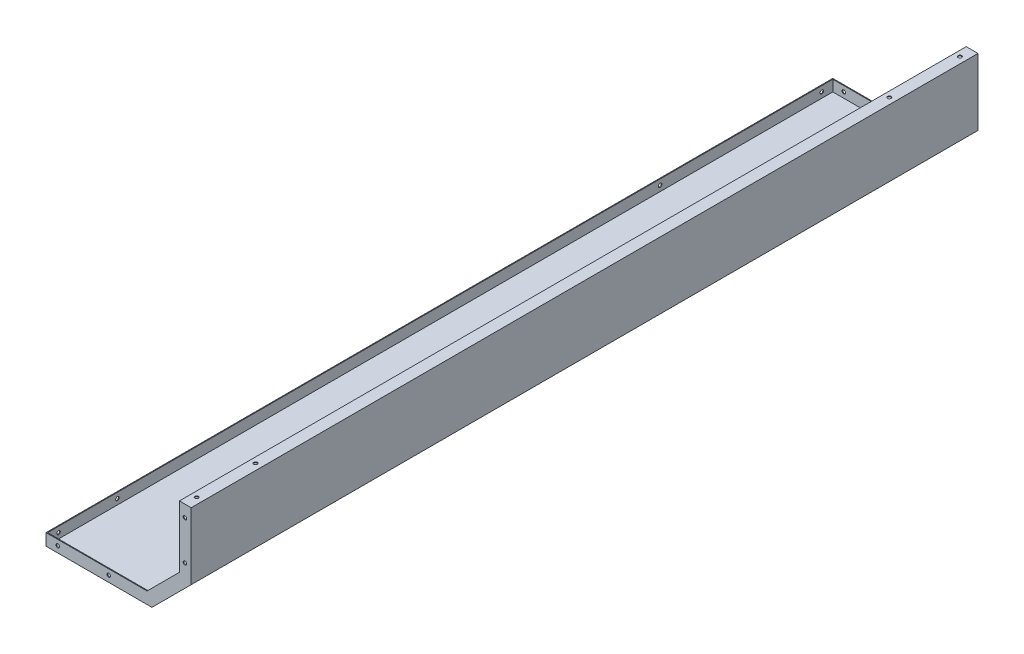
from build123d import *

# Parameters (mm, degrees)
EXTRUDE_1_DEPTH          = 2005
EXTRUDE_1_2_DEPTH        = 28
SKETCH_5_W               = 2
SKETCH_5_H               = 139.764501988
EXTRUDE_2_DEPTH          = 28
SKETCH_6_W               = 269.171572875
SKETCH_6_H               = 2
EXTRUDE_3_DEPTH          = 28
SKETCH_7_W               = 2
SKETCH_7_H               = 2005
EXTRUDE_4_DEPTH          = 28
CUT_EXTRUDE_1_DEPTH      = 10
CUT_EXTRUDE_1_DEPTH_BACK = 10
SKETCH_8_R               = 4.5
SKETCH_9_R               = 4.5
CUT_EXTRUDE_2_DEPTH      = 10
SKETCH_10_R              = 4.5
CUT_EXTRUDE_3_DEPTH      = 76
SKETCH_11_R              = 4.5
CUT_EXTRUDE_4_DEPTH      = 63
SKETCH_12_R              = 4.5
CUT_EXTRUDE_5_DEPTH      = 10
SKETCH_13_R              = 4.5
CUT_EXTRUDE_6_DEPTH      = 10


with BuildPart() as part:
    # 草图1 → Extrude 1 (new body)
    with BuildSketch(Plane.XY):
        Polygon((0, 0), (270, 0), (370, 100), (370, 270), (368, 270), (368, 100.828427125), (269.171572875, 2), (0, 2), align=None)
    extrude(amount=EXTRUDE_1_DEPTH)

    # 草图4 → Extrude 1 2 (add)
    with BuildSketch(Plane.ZY.offset(-368)):
        Polygon((0, 100.828427125), (0, 270), (2005, 270), (2005, 100.828427125), (2003, 100.828427125), (2003, 268), (2, 268), (2, 100.828427125), align=None)
    extrude(amount=EXTRUDE_1_2_DEPTH)

    # 草图5 → 凸台-拉伸2 (add)
    with BuildSketch(Plane(origin=(133.585786438, -133.585786438, 0), x_dir=(0, 0, 1), z_dir=(-0.7071067811865476, 0.7071067811865476, 0))):
        with Locations((1, 261.629509039)):
            Rectangle(SKETCH_5_W, SKETCH_5_H)
        with Locations((2004, 261.629509039)):
            Rectangle(SKETCH_5_W, SKETCH_5_H)
    extrude(amount=EXTRUDE_2_DEPTH)

    # 草图6 → 凸台-拉伸3 (add)
    with BuildSketch(Plane(origin=(0, 2, 0), x_dir=(1, 0, 0), z_dir=(0, 1, 0))):
        with Locations((134.585786438, -1)):
            Rectangle(SKETCH_6_W, SKETCH_6_H)
        with Locations((134.585786438, -2004)):
            Rectangle(SKETCH_6_W, SKETCH_6_H)
    extrude(amount=EXTRUDE_3_DEPTH)

    # 草图7 → 凸台-拉伸4 (add)
    with BuildSketch(Plane(origin=(0, 2, 0), x_dir=(1, 0, 0), z_dir=(0, 1, 0))):
        with Locations((1, -1002.5)):
            Rectangle(SKETCH_7_W, SKETCH_7_H)
    extrude(amount=EXTRUDE_4_DEPTH)

    # 草图8 → 切除-拉伸1 (cut, two sides: drawn at the far end of the back side and taken through both)
    with BuildSketch(Plane(origin=(0, 0, 2003), x_dir=(-1, 0, 0), z_dir=(0, 0, -1)).offset(-CUT_EXTRUDE_1_DEPTH_BACK)):
        with Locations(Location((-354, 240, 0), (0, 0, 180))):
            Circle(SKETCH_8_R)
        with Locations(Location((-30, 16, 0), (0, 0, 180))):
            Circle(SKETCH_8_R)
        with Locations(Location((-354, 140, 0), (0, 0, 180))):
            Circle(SKETCH_8_R)
        with Locations(Location((-160, 16, 0), (0, 0, 180))):
            Circle(SKETCH_8_R)
    extrude(amount=CUT_EXTRUDE_1_DEPTH + CUT_EXTRUDE_1_DEPTH_BACK, mode=Mode.SUBTRACT)

    # 草图9 → 切除-拉伸2 (cut)
    with BuildSketch(Plane.XZ.offset(-268)):
        with Locations(Location((354, 1975, 0), (0, 0, 270))):
            Circle(SKETCH_9_R)
        with Locations(Location((354, 1825, 0), (0, 0, 270))):
            Circle(SKETCH_9_R)
    extrude(amount=-CUT_EXTRUDE_2_DEPTH, mode=Mode.SUBTRACT)

    # 草图10 → 切除-拉伸3 (cut)
    with BuildSketch(Plane(origin=(2, 0, 0), x_dir=(0, 0, -1), z_dir=(1, 0, 0))):
        with Locations((-1975, 16)):
            Circle(SKETCH_10_R)
        with Locations((-1825, 16)):
            Circle(SKETCH_10_R)
    extrude(amount=-CUT_EXTRUDE_3_DEPTH, mode=Mode.SUBTRACT)

    # 草图11 → 切除-拉伸4 (cut)
    with BuildSketch(Plane.XZ.offset(-268)):
        with Locations(Location((354, 30, 0), (0, 0, 270))):
            Circle(SKETCH_11_R)
        with Locations(Location((354, 210, 0), (0, 0, 270))):
            Circle(SKETCH_11_R)
    extrude(amount=-CUT_EXTRUDE_4_DEPTH, mode=Mode.SUBTRACT)

    # 草图12 → 切除-拉伸5 (cut)
    with BuildSketch(Plane(origin=(2, 0, 0), x_dir=(0, 0, -1), z_dir=(1, 0, 0))):
        with Locations((-30, 16)):
            Circle(SKETCH_12_R)
        with Locations((-442, 16)):
            Circle(SKETCH_12_R)
    extrude(amount=-CUT_EXTRUDE_5_DEPTH, mode=Mode.SUBTRACT)

    # 草图13 → 切除-拉伸6 (cut)
    with BuildSketch(Plane(origin=(0, 0, 0), x_dir=(-1, 0, 0), z_dir=(0, 0, -1))):
        with Locations(Location((-30, 16, 0), (0, 0, 180))):
            Circle(SKETCH_13_R)
        with Locations(Location((-354, 240, 0), (0, 0, 180))):
            Circle(SKETCH_13_R)
        with Locations((-308.686291501, 61.313708499)):
            Circle(SKETCH_13_R)
    extrude(amount=-CUT_EXTRUDE_6_DEPTH, mode=Mode.SUBTRACT)


solid = part.part
